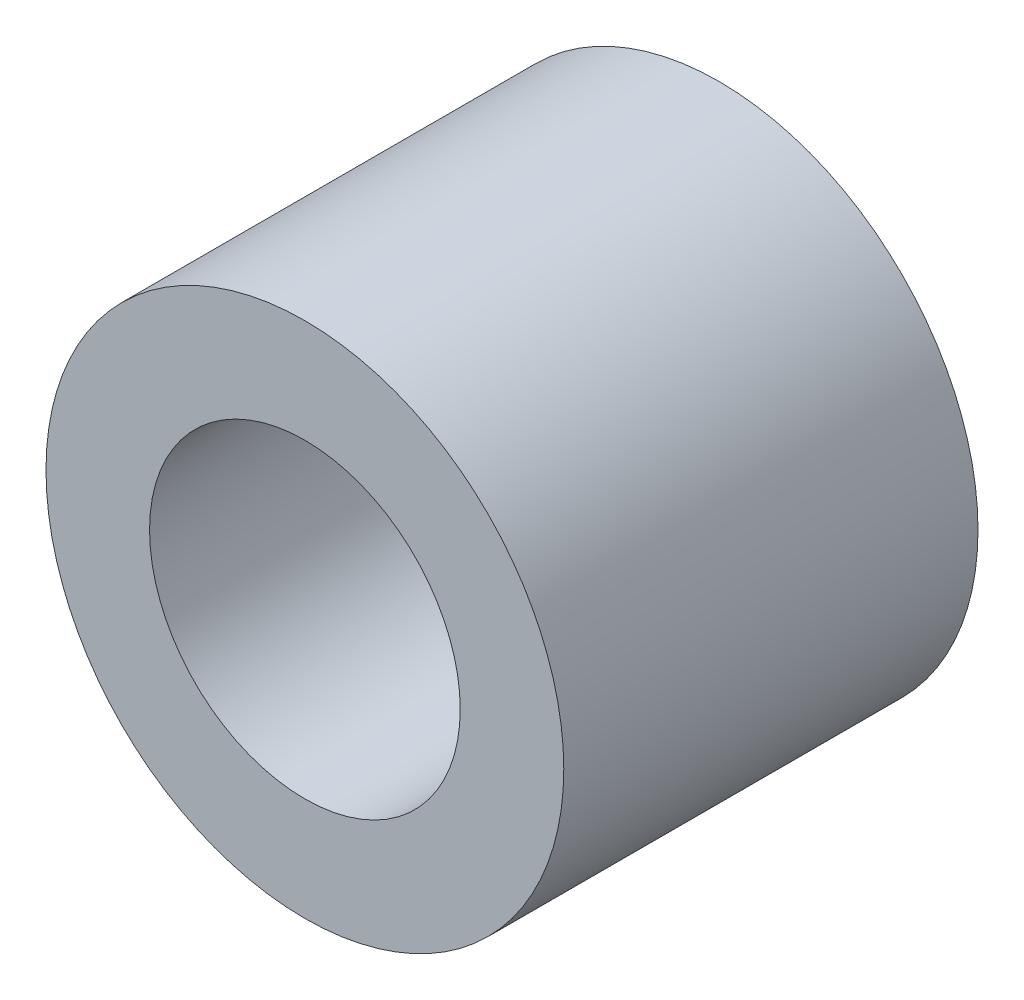
SolidWorks part; units mm, degrees
ref_plane "Front Plane" through (0, 0, 0) normal (0, 0, 1) x (1, 0, 0)
ref_plane "Top Plane" through (0, 0, 0) normal (0, 1, 0) x (1, 0, 0)
ref_plane "Right Plane" through (0, 0, 0) normal (1, 0, 0) x (0, 0, -1)
sketch "Sketch1" plane through (0, 0, 0) normal (0, 0, 1) x (1, 0, 0)
  circle A0 centre (0, 0) radius 25
  circle A1 centre (0, 0) radius 15
extrude "Boss-Extrude1" add sketch "Sketch1" along normal blind 40
